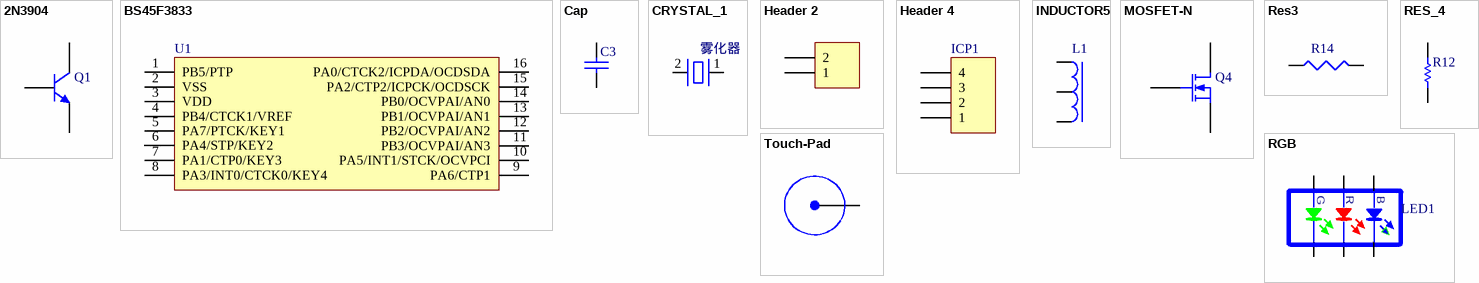
[diagram p0: symbols 2N3904 to Touch-Pad]
# Altium schematic symbol library MISC75988-4.SchLib: 12 symbols
Pins are listed as number, name and electrical type; pins without a type are passive.


## 2N3904
designator Q1
NPN General Purpose Amplifier
footprint TO-92A (TO, Flat Index; 3 In-Line, Axial Leads; Body Dia. 4.5mm; Leads 0.51 x 0.48 mm (max))
simulation model 2N3904 (NPN)
signal-integrity model 2N3904
pins: 1 E, 2 B, 3 C

## BS45F3833
designator U1
footprint NSOP 16
pins: 1 PB5/PTP, 2 VSS, 3 VDD, 4 PB4/CTCK1/VREF, 5 PA7/PTCK/KEY1, 6 PA4/STP/KEY2, 7 PA1/CTP0/KEY3, 8 PA3/INT0/CTCK0/KEY4, 9 PA6/CTP1, 10 PA5/INT1/STCK/OCVPCI, 11 PB3/OCVPAI/AN3, 12 PB2/OCVPAI/AN2, 13 PB1/OCVPAI/AN1, 14 PB0/OCVPAI/AN0, 15 PA2/CTP2/ICPCK/OCDSCK, 16 PA0/CTCK2/ICPDA/OCDSDA

## Cap
designator C3
Capacitor
footprint 0603C
pins: 1, 2

## CRYSTAL_1
designator 雾化器
footprint con2-wafer
pins: 1 OSC1, 2 OSC2

## Header 2
designator FAN1
Header, 2-Pin
footprint 2P/2.54MM
footprint con2-wafer
pins: 1, 2

## Header 4
designator ICP1
Header, 4-Pin
footprint HDR1X4 (Connector; Header; 4 Position)
signal-integrity model Connector
pins: 1, 2, 3, 4

## INDUCTOR5
designator L1
footprint TREE
pins: 1, 2, 3

## MOSFET-N
designator Q4
N-Channel MOSFET
footprint TO-252
footprint TO252-3 (D-PAK, 3-Pads, Body 5.7x6.7mm (max),)
pins: 1 D, 2 G, 3 S

## Res3
designator R14
Resistor
footprint 0603R
pins: 1, 2

## RES_4
designator R12
footprint 0603R
pins: 1, 2

## RGB
designator LED1
footprint LED-5050
pins: 1, 2, 3, 4, 5, 6

## Touch-Pad
designator WATER1
footprint Touch-Pad
pins: 1